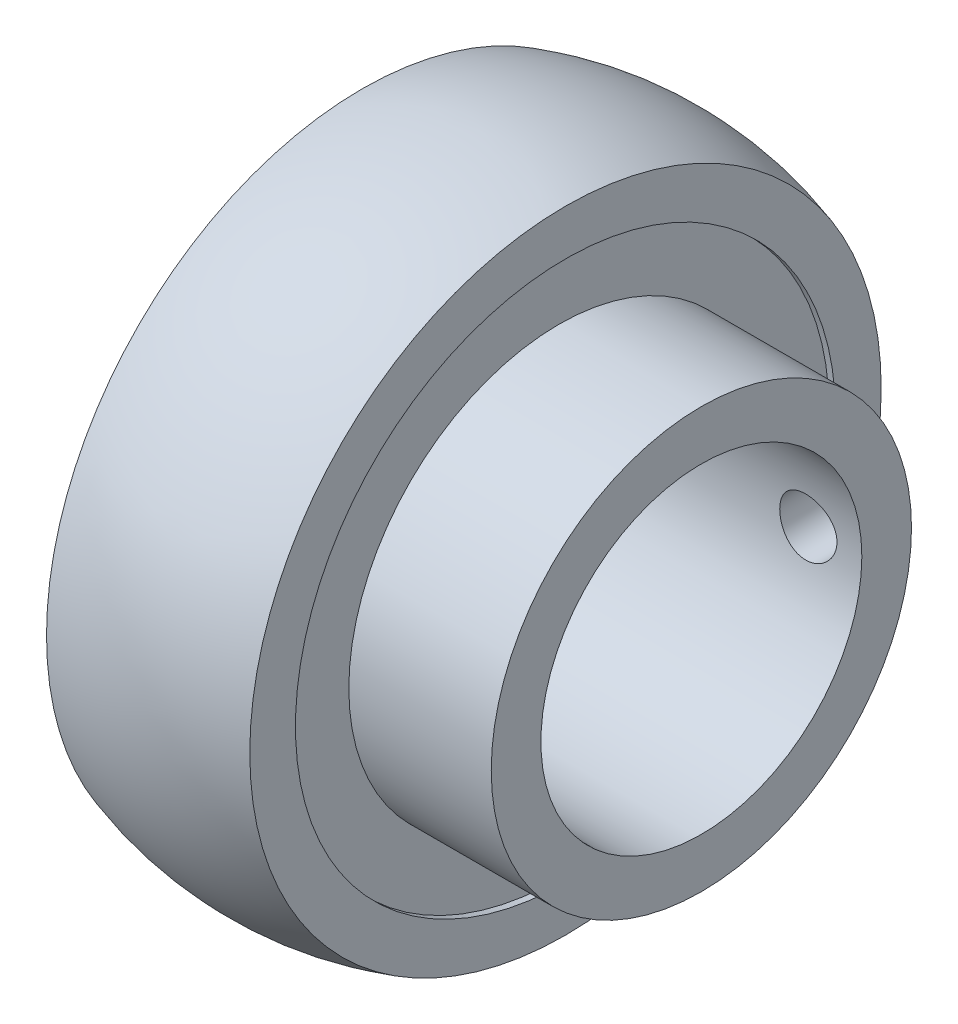
SolidWorks part; units mm, degrees
ref_plane "前视" through (0, 0, 0) normal (0, 0, 1) x (1, 0, 0)
ref_plane "上视" through (0, 0, 0) normal (0, 1, 0) x (1, 0, 0)
ref_plane "右视" through (0, 0, 0) normal (1, 0, 0) x (0, 0, -1)
sketch "尺寸草图" plane through (0, 0, 0) normal (0, 0, 1) x (1, 0, 0)
  line L0 (0, 0) -> (22.2, 0) construction
  line L2 (-15.9, 9.1908) -> (22.2, 9.1908)
  line L3 (-15.9, 9.1908) -> (-15.9, 15)
  line L4 (-15.9, 15) -> (22.2, 15)
  line L5 (22.2, 9.1908) -> (22.2, 15)
  arc A0 (-8, 30.4049) -> (8, 30.4049) centre (0, -23.0744) cw
  point P7 (0, 31)
  point P8 (17.2, 9.1908)
  point P12 (0, 31)
  point P13 (16.45, 9.1908)
  point P14 (22.45, 9.1908)
  point P15 (5, 30.7683)
  point P16 (7.5, 30.4774)
  dimension "d" = 30
  dimension "S" = 15.9
  dimension "B" = 38.1
  dimension "DD" = 62
  dimension "G" = 5
  dimension "C" = 16
  dimension "p" = 0.75
  dimension "ds" = 6
  dimension "Ca" = 5
  dimension "Cb" = 2.5
sketch "草图3" plane through (0, 0, 0) normal (1, 0, 0) x (0, 0, -1)
  line L0 (0, 0) -> (0, 23) construction
  line L1 (0, 18.44) -> (0, 27.56)
  arc A0 (0, 18.44) -> (0, 27.56) centre (0, 23) ccw
  dimension "D2" = 4.56
  dimension "D1" = 8
revolve "基体-旋转" add sketch "草图3" angle 360 about L0
sketch "草图2" plane through (0, 0, 0) normal (0, 0, 1) x (1, 0, 0)
  line L0 (-9.5, 25.24) -> (9.5, 25.24)
  line L1 (-15.9, 19.64) -> (22.2, 19.64)
  line L2 (-15.9, 19.64) -> (-15.9, 15)
  line L3 (-15.9, 15) -> (22.2, 15)
  line L4 (22.2, 19.64) -> (22.2, 15)
  line L5 (0, 0) -> (-6, 0) construction
  line L6 (9.5, 29.5085) -> (9.5, 25.24)
  line L7 (-9.5, 29.5085) -> (-9.5, 25.24)
  line L8 (0, 0) -> (0, 47.655) construction
  arc A1 (9.5, 29.5085) -> (-9.5, 29.5085) centre (0, 0) ccw
  dimension "D3" = 19
  dimension "D4" = 31
  dimension "D1" = 4.64
  dimension "D2" = 5.76
revolve "凸台-旋转3" add sketch "草图2" angle 360 about L5
pattern_circular "阵列(圆周)1" count 4 over 360 about axis through (0, 0, 0) along (1, 0, 0) of "基体-旋转"
sketch "草图5" plane through (0, 0, 0) normal (0, 0, 1) x (1, 0, 0)
  line L0 (-9.5, 29.5085) -> (-9.5, -29.5085) construction
  line L1 (-8.9, 25.74) -> (-8.7, 25.74)
  line L2 (-8.9, 25.74) -> (-8.9, 19.65)
  line L3 (-8.9, 19.65) -> (-8.7, 19.65)
  line L4 (-8.7, 25.74) -> (-8.7, 19.65)
  line L5 (0, 0) -> (-8.7, 0) construction
  line L6 (0, 0) -> (-6, 0) construction
  line L7 (0, 0) -> (0, 31) construction
  line L8 (8.7, 25.74) -> (8.7, 19.65)
  line L9 (-3.0829, 19.64) -> (-15.9, 19.64) construction
  line L11 (8.9, 19.65) -> (8.7, 19.65)
  line L12 (8.9, 25.74) -> (8.9, 19.65)
  line L13 (8.9, 25.74) -> (8.7, 25.74)
  line L15 (-3.9719, 25.24) -> (-9.5, 25.24) construction
  dimension "D1" = 0.5
  dimension "D2" = 0.01
  dimension "D3" = 0.2
  dimension "D4" = 0.6
revolve "凸台-旋转4" add sketch "草图5" angle 360 about L5
sketch "草图4" plane through (0, 0, 0) normal (0, 1, 0) x (1, 0, 0)
  line L0 (17.2, 19.94) -> (17.2, 13) construction
  line L1 (17.2, 19.94) -> (19.8753, 19.94)
  line L2 (22.2, 15) -> (-15.9, 15) construction
  line L3 (17.2, 13) -> (19.8753, 13)
  line L4 (19.8753, 19.94) -> (19.8753, 13)
  line L6 (22.2, -19.64) -> (22.2, 19.64) construction
  line L7 (17.2, 19.94) -> (17.2, 13)
  line L8 (22.2, 19.64) -> (3.0829, 19.64) construction
  dimension "D1" = 2
  dimension "D2" = 0.3
  dimension "D3" = 5
  dimension "D4" = 5.3505
revolve "切除-旋转1" cut sketch "草图4" angle 360 about L0
cosmetic thread "装饰螺纹线1" parameters "D2"=6
sketch "草图6" plane through (0, 0, 0) normal (0, 1, 0) x (1, 0, 0)
  line L0 (0, 0) -> (0, 31) construction
  line L1 (5, 31.5) -> (5, 24.74) construction
  line L2 (5, 31.5) -> (6.25, 31.5)
  line L3 (6.25, 31.5) -> (6.25, 24.74)
  line L4 (6.25, 24.74) -> (5, 24.74)
  line L5 (8.7, 25.24) -> (3.9719, 25.24) construction
  line L6 (5, 31.5) -> (5, 24.74)
  dimension "D1" = 5
  dimension "D2" = 2.5
  dimension "D3" = 0.5
  dimension "D4" = 0.5
  dimension "D5" = 31
revolve "切除-旋转2" cut sketch "草图6" angle 360 about L1
